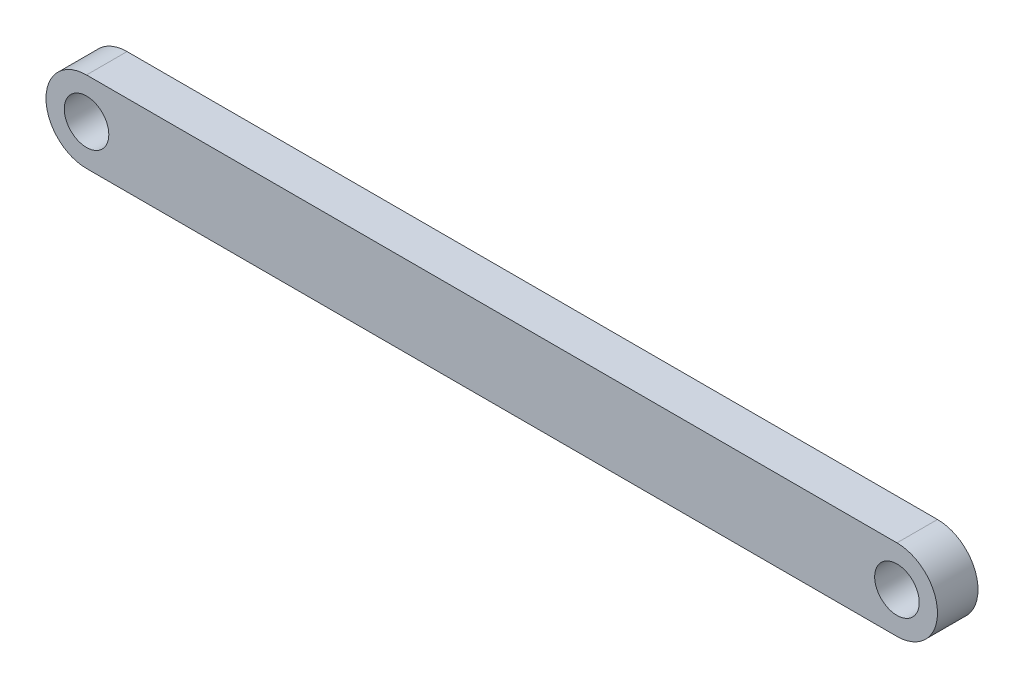
SolidWorks part; units mm, degrees
ref_plane "Alzado" through (0, 0, 0) normal (0, 0, 1) x (1, 0, 0)
ref_plane "Planta" through (0, 0, 0) normal (0, 1, 0) x (1, 0, 0)
ref_plane "Vista lateral" through (0, 0, 0) normal (1, 0, 0) x (0, 0, -1)
sketch "Sketch1" plane through (0, 0, 0) normal (0, 0, 1) x (1, 0, 0)
  line L0 (-10, 0) -> (10, 0) construction
  line L1 (-10, 1) -> (10, 1)
  line L2 (-10, -1) -> (10, -1)
  arc A0 (-10, 1) -> (-10, -1) centre (-10, 0) ccw
  arc A1 (10, -1) -> (10, 1) centre (10, 0) ccw
  circle A2 centre (-10, 0) radius 0.55
  circle A3 centre (10, 0) radius 0.55
  point P3 (0, 0)
  dimension "D3" = 1.1
  dimension "D1" = 20
  dimension "D2" = 2
extrude "Thigh1 length" add sketch "Sketch1" along normal mid plane 1
sketch "Sketch2" plane through (0, 0, 0.5) normal (0, 0, 1) x (1, 0, 0)
  circle A0 centre (-10, 0) radius 1.55
  circle A1 centre (10, 0) radius 1.55
  dimension "D1" = 3.1
extrude "Cortar-Extruir1" [suppressed] cut sketch "Sketch2" against normal blind 0.5
